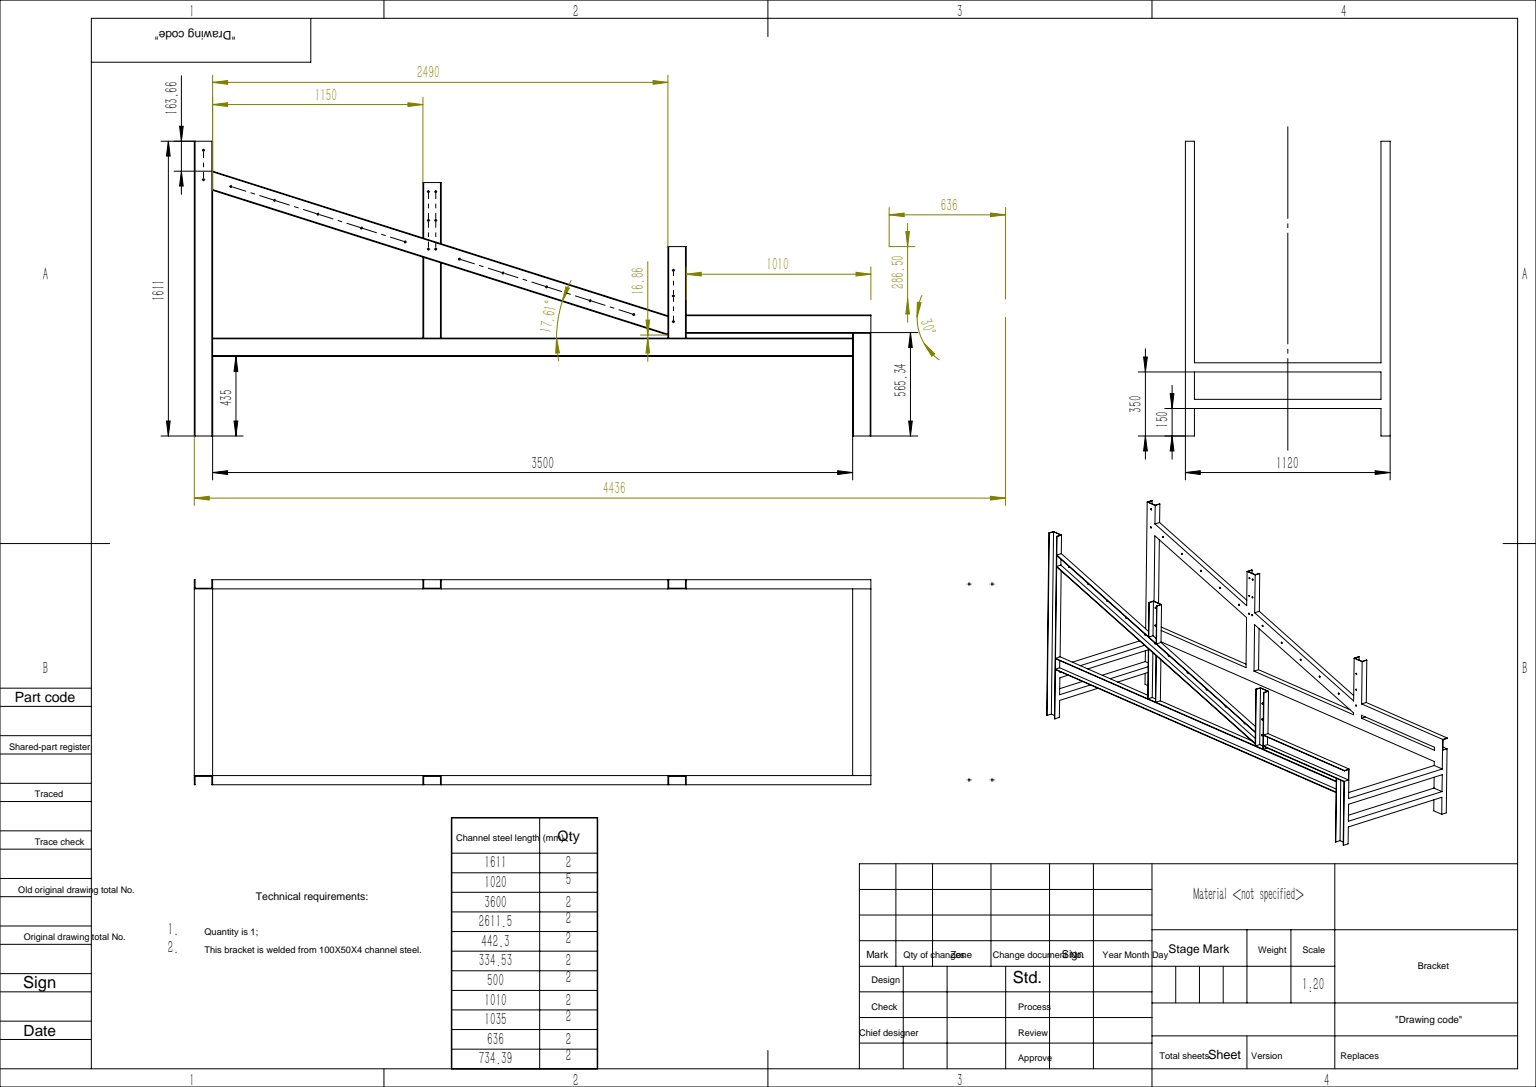
from build123d import *

# Parameters (mm, degrees)
EXTRUDE_1_DEPTH             = 1611
EXTRUDE_1_2_DEPTH           = 1611
EXTRUDE_2_DEPTH             = 3500
EXTRUDE_3_DEPTH             = 535
EXTRUDE_6_DEPTH             = 500
EXTRUDE_7_DEPTH             = 850
EXTRUDE_5_REACH             = 4313.074
EXTRUDE_5_DIRECTION_2_REACH = 4313.074
EXTRUDE_8_DEPTH             = 1020
SKETCH_22_W                 = 46
SKETCH_22_H                 = 92
CUT_EXTRUDE_5_DEPTH         = 1500
EXTRUDE_9_DEPTH             = 1010
EXTRUDE_4_DEPTH             = 26.339444378
SKETCH_20_R                 = 5
CUT_EXTRUDE_3_DEPTH         = 4176.978567953
PATTERN_LINEAR_1_COUNT      = 2
PATTERN_LINEAR_1_PITCH      = 160
SKETCH_21_R                 = 5
CUT_EXTRUDE_4_DEPTH         = 4176.978567953
PATTERN_LINEAR_2_COUNT      = 5
PATTERN_LINEAR_2_PITCH      = 250
SKETCH_23_R                 = 5
CUT_EXTRUDE_6_DEPTH         = 4176.978567953
PATTERN_LINEAR_3_COUNT      = 3
PATTERN_LINEAR_3_PITCH      = 157
SKETCH_24_R                 = 5
CUT_EXTRUDE_7_DEPTH         = 4176.978567953
PATTERN_LINEAR_4_COUNT      = 5
PATTERN_LINEAR_4_PITCH      = 250
SKETCH_25_R                 = 5
CUT_EXTRUDE_8_DEPTH         = 4176.978567953
PATTERN_LINEAR_5_COUNT      = 3
PATTERN_LINEAR_5_PITCH      = 140
PATTERN_LINEAR_8_COUNT      = 2
PATTERN_LINEAR_8_PITCH      = 200
PATTERN_LINEAR_8_COUNT_DIR2 = 2
PATTERN_LINEAR_8_PITCH_DIR2 = 3600
MIRROR_7_COPY_1_SKETCH_R    = 5
MIRROR_7_COPY_1_DEPTH       = 4176.978567953
MIRROR_7_COPY_2_SKETCH_R    = 5
MIRROR_7_COPY_2_DEPTH       = 4176.978567953
MIRROR_7_COPY_3_SKETCH_R    = 5
MIRROR_7_COPY_3_DEPTH       = 4176.978567953
MIRROR_7_COPY_4_SKETCH_R    = 5
MIRROR_7_COPY_4_DEPTH       = 4176.978567953
MIRROR_7_COPY_5_SKETCH_R    = 5
MIRROR_7_COPY_5_DEPTH       = 4176.978567953
MIRROR_7_COPY_6_SKETCH_R    = 5
MIRROR_7_COPY_6_DEPTH       = 4176.978567953
MIRROR_7_COPY_7_SKETCH_R    = 5
MIRROR_7_COPY_7_DEPTH       = 4176.978567953
MIRROR_7_COPY_8_SKETCH_R    = 5
MIRROR_7_COPY_8_DEPTH       = 4176.978567953
MIRROR_7_COPY_9_SKETCH_R    = 5
MIRROR_7_COPY_9_DEPTH       = 4176.978567953
MIRROR_7_COPY_10_SKETCH_R   = 5
MIRROR_7_COPY_10_DEPTH      = 4176.978567953
MIRROR_7_COPY_11_SKETCH_R   = 5
MIRROR_7_COPY_11_DEPTH      = 4176.978567953
MIRROR_7_COPY_12_SKETCH_R   = 5
MIRROR_7_COPY_12_DEPTH      = 4176.978567953
MIRROR_7_COPY_13_SKETCH_R   = 5
MIRROR_7_COPY_13_DEPTH      = 4176.978567953


with BuildPart() as part:
    # 草图1 → 凸台-拉伸1 (new body)
    with BuildSketch(Plane(origin=(0, 0, 0), x_dir=(1, 0, 0), z_dir=(0, 1, 0))):
        Polygon((0, -560), (4, -560), (4, -514), (96, -514), (96, -560), (100, -560), (100, -510), (0, -510), align=None)
    extrude(amount=EXTRUDE_1_DEPTH)



with BuildPart() as body_2:
    # 草图1 → Extrude 1 2 (new body)
    with BuildSketch(Plane(origin=(0, 0, 0), x_dir=(1, 0, 0), z_dir=(0, 1, 0))):
        Polygon((96, 560), (100, 560), (100, 510), (0, 510), (0, 560), (4, 560), (4, 514), (96, 514), align=None)
    extrude(amount=EXTRUDE_1_2_DEPTH)


with BuildPart() as part_1:
    add(part.part)

    add(body_2.part)  # 凸台-拉伸2 merges body 2
    # 草图2 → 凸台-拉伸2 (add)
    with BuildSketch(Plane(origin=(100, 0, 0), x_dir=(0, 0, -1), z_dir=(1, 0, 0))):
        Polygon((-560, 535), (-510, 535), (-510, 435), (-560, 435), (-560, 439), (-514, 439), (-514, 531), (-560, 531), align=None)
        Polygon((560, 435), (510, 435), (510, 535), (560, 535), (560, 531), (514, 531), (514, 439), (560, 439), align=None)
    extrude(amount=EXTRUDE_2_DEPTH)

    # 草图4 → 凸台-拉伸3 (add)
    with BuildSketch(Plane(origin=(0, 535, 0), x_dir=(1, 0, 0), z_dir=(0, 1, 0))):
        Polygon((3604, -560), (3604, -514), (3696, -514), (3696, -560), (3700, -560), (3700, -510), (3600, -510), (3600, -560), align=None)
        Polygon((3696, 560), (3700, 560), (3700, 510), (3600, 510), (3600, 560), (3604, 560), (3604, 514), (3696, 514), align=None)
    extrude(amount=-EXTRUDE_3_DEPTH)

    # 草图9 → 凸台-拉伸6 (add)
    with BuildSketch(Plane(origin=(0, 535, 0), x_dir=(1, 0, 0), z_dir=(0, 1, 0))):
        Polygon((2690, 560), (2686, 560), (2686, 514), (2594, 514), (2594, 560), (2590, 560), (2590, 510), (2690, 510), align=None)
    extrude_6 = extrude(amount=EXTRUDE_6_DEPTH)

    # 草图10 → 凸台-拉伸7 (add)
    with BuildSketch(Plane(origin=(0, 535, 0), x_dir=(1, 0, 0), z_dir=(0, 1, 0))):
        Polygon((1346, 560), (1346, 514), (1254, 514), (1254, 560), (1250, 560), (1250, 510), (1350, 510), (1350, 560), align=None)
    extrude_7 = extrude(amount=EXTRUDE_7_DEPTH)

    # 凸台-拉伸5: up to this face of the body (flat: up to its plane)
    extrude_5_end = Plane(part_1.part.faces().sort_by_distance((2590, 785, -535))[0])
    # 草图8 → 凸台-拉伸5 (add, up to the picked face)
    with BuildSketch(Plane(origin=(-296.339746708, 94.086464687, 0), x_dir=(0, 0, -1), z_dir=(0.9531146620938385, -0.30260938667157716, 0)), mode=Mode.PRIVATE) as extrude_5_sk1:
        Polygon((560, 1405.740425), (514, 1405.740425), (514, 1313.740425), (560, 1313.740425), (560, 1309.740425), (510, 1309.740425), (510, 1409.740425), (560, 1409.740425), align=None)
    extrude_5_tool1 = split(extrude(extrude_5_sk1.sketch, amount=EXTRUDE_5_REACH, mode=Mode.PRIVATE), bisect_by=extrude_5_end, keep=Keep.BOTH, mode=Mode.PRIVATE)
    extrude_5 = extrude_5_tool1.solids().sort_by(Axis((129.388829, 1434.983889, -537), (0.9531146620938385, -0.30260938667157716, 0)))[0]
    add(extrude_5)

    # 凸台-拉伸5 direction 2: up to this face of the body (flat: up to its plane)
    extrude_5_direction_2_end = Plane(part_1.part.faces().sort_by_distance((100, 1073, -535))[0])
    # 草图8 → 凸台-拉伸5 direction 2 (add, up to the picked face)
    with BuildSketch(Plane(origin=(-296.339746708, 94.086464687, 0), x_dir=(0, 0, -1), z_dir=(0.9531146620938385, -0.30260938667157716, 0)), mode=Mode.PRIVATE) as extrude_5_direction_2_sk1:
        Polygon((560, 1405.740425), (514, 1405.740425), (514, 1313.740425), (560, 1313.740425), (560, 1309.740425), (510, 1309.740425), (510, 1409.740425), (560, 1409.740425), align=None)
    extrude_5_direction_2_tool1 = split(extrude(extrude_5_direction_2_sk1.sketch, amount=-EXTRUDE_5_DIRECTION_2_REACH, mode=Mode.PRIVATE), bisect_by=extrude_5_direction_2_end, keep=Keep.BOTH, mode=Mode.PRIVATE)
    extrude_5_direction_2 = extrude_5_direction_2_tool1.solids().sort_by(Axis((129.388829, 1434.983889, -537), (-0.9531146620938385, 0.30260938667157716, 0)))[0]
    add(extrude_5_direction_2)

    # 草图12 → 凸台-拉伸8 (add)
    with BuildSketch(Plane.XY.offset(-510)):
        Polygon((3600, 400), (3700, 400), (3700, 350), (3696, 350), (3696, 396), (3604, 396), (3604, 350), (3600, 350), align=None)
    extrude_8 = extrude(amount=EXTRUDE_8_DEPTH)

    # 草图22 → 切除-拉伸5 (cut)
    with BuildSketch(Plane(origin=(-296.339746708, 94.086464687, 0), x_dir=(0, 0, -1), z_dir=(0.9531146620938385, -0.30260938667157716, 0))):
        with Locations((537, 1359.740425)):
            Rectangle(SKETCH_22_W, SKETCH_22_H)
    cut_extrude_5 = extrude(amount=CUT_EXTRUDE_5_DEPTH, mode=Mode.SUBTRACT)

    # 草图30 → 凸台-拉伸9 (add)
    with BuildSketch(Plane(origin=(2690, 0, 0), x_dir=(0, 0, -1), z_dir=(1, 0, 0))):
        Polygon((560, 657.339444378), (514, 657.339444378), (514, 565.339444378), (560, 565.339444378), (560, 561.339444378), (510, 561.339444378), (510, 661.339444378), (560, 661.339444378), align=None)
    extrude_9 = extrude(amount=EXTRUDE_9_DEPTH)

    # 草图5 → 凸台-拉伸4 (add)
    with BuildSketch(Plane(origin=(0, 535, 0), x_dir=(1, 0, 0), z_dir=(0, 1, 0))):
        Polygon((3600, 560), (3600, 510), (3700, 510), (3700, 560), (3696, 560), (3696, 514), (3604, 514), (3604, 560), align=None)
    extrude_4 = extrude(amount=EXTRUDE_4_DEPTH)

    # 草图20 → 切除-拉伸3 (cut, through all)
    with BuildSketch(Plane(origin=(0, 0, -514), x_dir=(-1, 0, 0), z_dir=(0, 0, -1))):
        with Locations((-50, 1561)):
            Circle(SKETCH_20_R)
    cut_extrude_3 = extrude(amount=-CUT_EXTRUDE_3_DEPTH, mode=Mode.SUBTRACT)

    # 阵列(线性)1: 切除-拉伸3 ×2
    with Locations(*[(0, -i * PATTERN_LINEAR_1_PITCH, 0) for i in range(1, PATTERN_LINEAR_1_COUNT)]):
        add(cut_extrude_3, mode=Mode.SUBTRACT)

    # 草图21 → 切除-拉伸4 (cut, through all)
    with BuildSketch(Plane(origin=(0, 0, -514), x_dir=(-1, 0, 0), z_dir=(0, 0, -1))):
        with Locations((-200, 1363.129326761)):
            Circle(SKETCH_21_R)
    cut_extrude_4 = extrude(amount=-CUT_EXTRUDE_4_DEPTH, mode=Mode.SUBTRACT)

    # 阵列(线性)2: 切除-拉伸4 ×5
    with Locations(*[Vector(0.9531146620938384, -0.3026093866715778, 0) * (i * PATTERN_LINEAR_2_PITCH) for i in range(1, PATTERN_LINEAR_2_COUNT)]):
        add(cut_extrude_4, mode=Mode.SUBTRACT)

    # 草图23 → 切除-拉伸6 (cut, through all)
    with BuildSketch(Plane(origin=(0, 0, -514), x_dir=(-1, 0, 0), z_dir=(0, 0, -1))):
        with Locations(Location((-1280, 1335, 0), (0, 0, 90))):
            Circle(SKETCH_23_R)
        with Locations(Location((-1320, 1335, 0), (0, 0, 90))):
            Circle(SKETCH_23_R)
    cut_extrude_6 = extrude(amount=-CUT_EXTRUDE_6_DEPTH, mode=Mode.SUBTRACT)

    # 阵列(线性)3: 切除-拉伸6 ×3
    with Locations(*[(0, -i * PATTERN_LINEAR_3_PITCH, 0) for i in range(1, PATTERN_LINEAR_3_COUNT)]):
        add(cut_extrude_6, mode=Mode.SUBTRACT)

    # 草图24 → 切除-拉伸7 (cut, through all)
    with BuildSketch(Plane(origin=(0, 0, -514), x_dir=(-1, 0, 0), z_dir=(0, 0, -1))):
        with Locations((-1450, 966.260252783)):
            Circle(SKETCH_24_R)
    cut_extrude_7 = extrude(amount=-CUT_EXTRUDE_7_DEPTH, mode=Mode.SUBTRACT)

    # 阵列(线性)4: 切除-拉伸7 ×5
    with Locations(*[Vector(0.9531146620938387, -0.3026093866715769, 0) * (i * PATTERN_LINEAR_4_PITCH) for i in range(1, PATTERN_LINEAR_4_COUNT)]):
        add(cut_extrude_7, mode=Mode.SUBTRACT)

    # 草图25 → 切除-拉伸8 (cut, through all)
    with BuildSketch(Plane(origin=(0, 0, -514), x_dir=(-1, 0, 0), z_dir=(0, 0, -1))):
        with Locations(Location((-2620, 905, 0), (0, 0, 90))):
            Circle(SKETCH_25_R)
    cut_extrude_8 = extrude(amount=-CUT_EXTRUDE_8_DEPTH, mode=Mode.SUBTRACT)

    # 阵列(线性)5: 切除-拉伸8 ×3
    with Locations(*[(0, -i * PATTERN_LINEAR_5_PITCH, 0) for i in range(1, PATTERN_LINEAR_5_COUNT)]):
        add(cut_extrude_8, mode=Mode.SUBTRACT)

    # 阵列(线性)8: Extrude 8 2 × 2
    with Locations(*[(-j * PATTERN_LINEAR_8_PITCH_DIR2, -i * PATTERN_LINEAR_8_PITCH, 0) for i in range(PATTERN_LINEAR_8_COUNT) for j in range(PATTERN_LINEAR_8_COUNT_DIR2) if (i, j) != (0, 0)]):
        add(extrude_8)

    # 镜向7: 凸台-拉伸6, 凸台-拉伸7, 凸台-拉伸5, 凸台-拉伸5 direction 2, 切除-拉伸5, 凸台-拉伸9, 凸台-拉伸4, 切除-拉伸3, 切除-拉伸4, 切除-拉伸6, 切除-拉伸7, 切除-拉伸8 across plane
    add(extrude_6.mirror(Plane.XY))
    add(extrude_7.mirror(Plane.XY))
    add(extrude_5.mirror(Plane.XY))
    add(extrude_5_direction_2.mirror(Plane.XY))
    add(cut_extrude_5.mirror(Plane.XY), mode=Mode.SUBTRACT)
    add(extrude_9.mirror(Plane.XY))
    add(extrude_4.mirror(Plane.XY))
    add(cut_extrude_3.mirror(Plane.XY), mode=Mode.SUBTRACT)
    add(cut_extrude_4.mirror(Plane.XY), mode=Mode.SUBTRACT)
    add(cut_extrude_6.mirror(Plane.XY), mode=Mode.SUBTRACT)
    add(cut_extrude_7.mirror(Plane.XY), mode=Mode.SUBTRACT)
    add(cut_extrude_8.mirror(Plane.XY), mode=Mode.SUBTRACT)

    # 镜向7 copy 1 sketch → 镜向7 copy 1 (cut, through all)
    with BuildSketch(Plane(origin=(0, -160, 514), x_dir=(-1, 0, 0), z_dir=(0, 0, 1))):
        with Locations((-50, -1561)):
            Circle(MIRROR_7_COPY_1_SKETCH_R)
    extrude(amount=-MIRROR_7_COPY_1_DEPTH, mode=Mode.SUBTRACT)

    # 镜向7 copy 2 sketch → 镜向7 copy 2 (cut, through all)
    with BuildSketch(Plane(origin=(238.278665523, -75.652346668, 514), x_dir=(-1, 0, 0), z_dir=(0, 0, 1))):
        with Locations((-200, -1363.129326761)):
            Circle(MIRROR_7_COPY_2_SKETCH_R)
    extrude(amount=-MIRROR_7_COPY_2_DEPTH, mode=Mode.SUBTRACT)

    # 镜向7 copy 3 sketch → 镜向7 copy 3 (cut, through all)
    with BuildSketch(Plane(origin=(476.557331047, -151.304693336, 514), x_dir=(-1, 0, 0), z_dir=(0, 0, 1))):
        with Locations((-200, -1363.129326761)):
            Circle(MIRROR_7_COPY_3_SKETCH_R)
    extrude(amount=-MIRROR_7_COPY_3_DEPTH, mode=Mode.SUBTRACT)

    # 镜向7 copy 4 sketch → 镜向7 copy 4 (cut, through all)
    with BuildSketch(Plane(origin=(714.83599657, -226.957040004, 514), x_dir=(-1, 0, 0), z_dir=(0, 0, 1))):
        with Locations((-200, -1363.129326761)):
            Circle(MIRROR_7_COPY_4_SKETCH_R)
    extrude(amount=-MIRROR_7_COPY_4_DEPTH, mode=Mode.SUBTRACT)

    # 镜向7 copy 5 sketch → 镜向7 copy 5 (cut, through all)
    with BuildSketch(Plane(origin=(953.114662094, -302.609386672, 514), x_dir=(-1, 0, 0), z_dir=(0, 0, 1))):
        with Locations((-200, -1363.129326761)):
            Circle(MIRROR_7_COPY_5_SKETCH_R)
    extrude(amount=-MIRROR_7_COPY_5_DEPTH, mode=Mode.SUBTRACT)

    # 镜向7 copy 6 sketch → 镜向7 copy 6 (cut, through all)
    with BuildSketch(Plane(origin=(0, -157, 514), x_dir=(-1, 0, 0), z_dir=(0, 0, 1))):
        with Locations((-1280, -1335)):
            Circle(MIRROR_7_COPY_6_SKETCH_R)
        with Locations((-1320, -1335)):
            Circle(MIRROR_7_COPY_6_SKETCH_R)
    extrude(amount=-MIRROR_7_COPY_6_DEPTH, mode=Mode.SUBTRACT)

    # 镜向7 copy 7 sketch → 镜向7 copy 7 (cut, through all)
    with BuildSketch(Plane(origin=(0, -314, 514), x_dir=(-1, 0, 0), z_dir=(0, 0, 1))):
        with Locations((-1280, -1335)):
            Circle(MIRROR_7_COPY_7_SKETCH_R)
        with Locations((-1320, -1335)):
            Circle(MIRROR_7_COPY_7_SKETCH_R)
    extrude(amount=-MIRROR_7_COPY_7_DEPTH, mode=Mode.SUBTRACT)

    # 镜向7 copy 8 sketch → 镜向7 copy 8 (cut, through all)
    with BuildSketch(Plane(origin=(238.278665523, -75.652346668, 514), x_dir=(-1, 0, 0), z_dir=(0, 0, 1))):
        with Locations((-1450, -966.260252783)):
            Circle(MIRROR_7_COPY_8_SKETCH_R)
    extrude(amount=-MIRROR_7_COPY_8_DEPTH, mode=Mode.SUBTRACT)

    # 镜向7 copy 9 sketch → 镜向7 copy 9 (cut, through all)
    with BuildSketch(Plane(origin=(476.557331047, -151.304693336, 514), x_dir=(-1, 0, 0), z_dir=(0, 0, 1))):
        with Locations((-1450, -966.260252783)):
            Circle(MIRROR_7_COPY_9_SKETCH_R)
    extrude(amount=-MIRROR_7_COPY_9_DEPTH, mode=Mode.SUBTRACT)

    # 镜向7 copy 10 sketch → 镜向7 copy 10 (cut, through all)
    with BuildSketch(Plane(origin=(714.83599657, -226.957040004, 514), x_dir=(-1, 0, 0), z_dir=(0, 0, 1))):
        with Locations((-1450, -966.260252783)):
            Circle(MIRROR_7_COPY_10_SKETCH_R)
    extrude(amount=-MIRROR_7_COPY_10_DEPTH, mode=Mode.SUBTRACT)

    # 镜向7 copy 11 sketch → 镜向7 copy 11 (cut, through all)
    with BuildSketch(Plane(origin=(953.114662094, -302.609386672, 514), x_dir=(-1, 0, 0), z_dir=(0, 0, 1))):
        with Locations((-1450, -966.260252783)):
            Circle(MIRROR_7_COPY_11_SKETCH_R)
    extrude(amount=-MIRROR_7_COPY_11_DEPTH, mode=Mode.SUBTRACT)

    # 镜向7 copy 12 sketch → 镜向7 copy 12 (cut, through all)
    with BuildSketch(Plane(origin=(0, -140, 514), x_dir=(-1, 0, 0), z_dir=(0, 0, 1))):
        with Locations((-2620, -905)):
            Circle(MIRROR_7_COPY_12_SKETCH_R)
    extrude(amount=-MIRROR_7_COPY_12_DEPTH, mode=Mode.SUBTRACT)

    # 镜向7 copy 13 sketch → 镜向7 copy 13 (cut, through all)
    with BuildSketch(Plane(origin=(0, -280, 514), x_dir=(-1, 0, 0), z_dir=(0, 0, 1))):
        with Locations((-2620, -905)):
            Circle(MIRROR_7_COPY_13_SKETCH_R)
    extrude(amount=-MIRROR_7_COPY_13_DEPTH, mode=Mode.SUBTRACT)


solid = part_1.part
